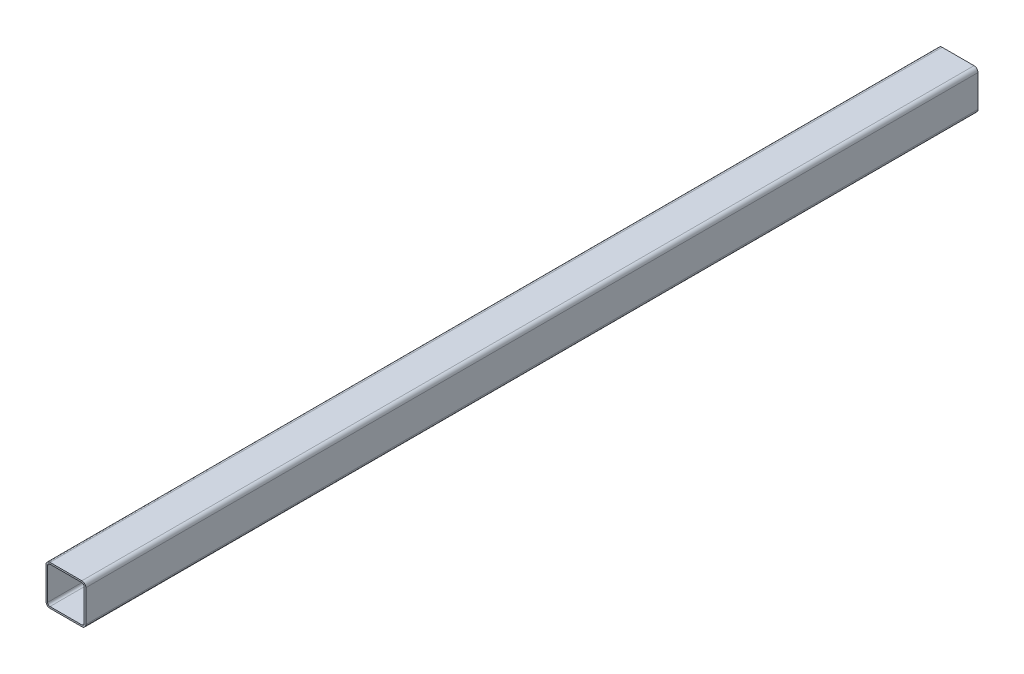
from build123d import *

# Parameters (mm, degrees)
BOSS_EXTRUDE1_DEPTH = 4480


with BuildPart() as part:
    # Sketch1 → Boss-Extrude1 (new body)
    with BuildSketch(Plane.XY):
        with BuildLine():
            Line((-80, 100), (80, 100))
            ThreePointArc((80, 100), (94.142135624, 94.142135624), (100, 80))
            Line((100, 80), (100, -80))
            ThreePointArc((100, -80), (94.142135624, -94.142135624), (80, -100))
            Line((80, -100), (-80, -100))
            ThreePointArc((-80, -100), (-94.142135624, -94.142135624), (-100, -80))
            Line((-100, -80), (-100, 80))
            ThreePointArc((-100, 80), (-94.142135624, 94.142135624), (-80, 100))
        make_face()
        with BuildLine():
            Line((-92, 80), (-92, -80))
            ThreePointArc((-92, -80), (-88.485281374, -88.485281374), (-80, -92))
            Line((-80, -92), (80, -92))
            ThreePointArc((80, -92), (88.485281374, -88.485281374), (92, -80))
            Line((92, -80), (92, 80))
            ThreePointArc((92, 80), (88.485281374, 88.485281374), (80, 92))
            Line((80, 92), (-80, 92))
            ThreePointArc((-80, 92), (-88.485281374, 88.485281374), (-92, 80))
        make_face(mode=Mode.SUBTRACT)
    extrude(amount=BOSS_EXTRUDE1_DEPTH)


solid = part.part
